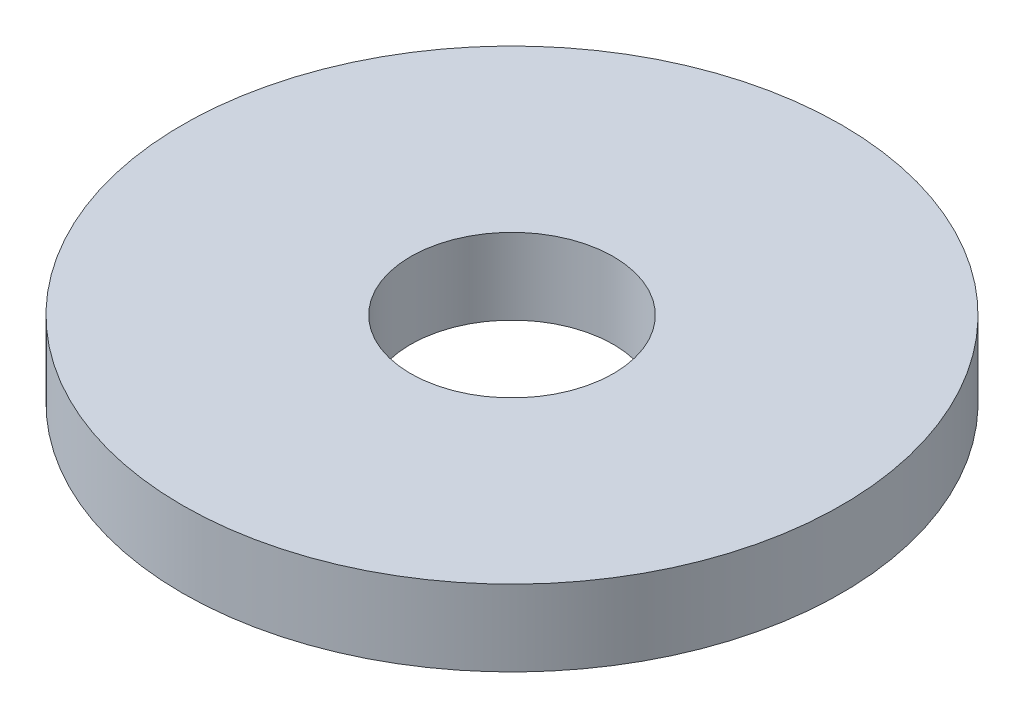
SolidWorks part; units mm, degrees
ref_plane "前视基准面" through (0, 0, 0) normal (0, 0, 1) x (1, 0, 0)
ref_plane "上视基准面" through (0, 0, 0) normal (0, 1, 0) x (1, 0, 0)
ref_plane "右视基准面" through (0, 0, 0) normal (1, 0, 0) x (0, 0, -1)
sketch "草图1" plane through (0, 0, 0) normal (0, 1, 0) x (1, 0, 0)
  circle A0 centre (0, 0) radius 20
  circle A1 centre (0, 0) radius 65
  dimension "D1" = 40
  dimension "D2" = 130
extrude "凸台-拉伸1" add sketch "草图1" along normal mid plane 15
